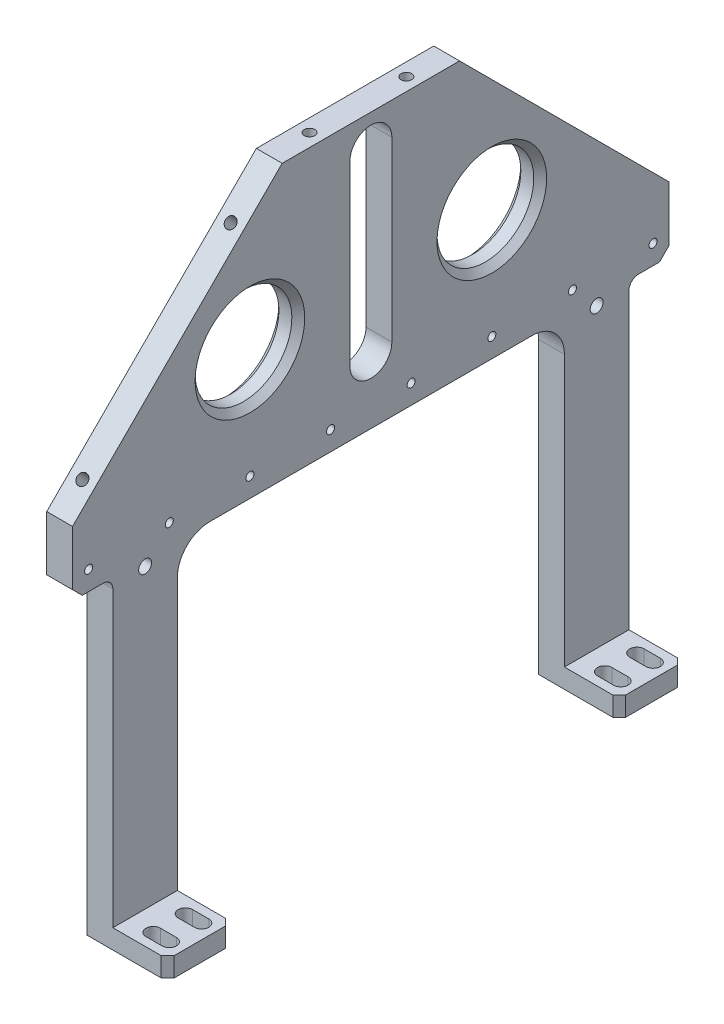
from build123d import *

# Parameters (mm, degrees)
BOSS_EXTRUDE1_DEPTH        = 92.5
CUT_EXTRUDE5_DEPTH         = 209.3416665
M4_TAPPED_HOLE1_D          = 3.3
M4_TAPPED_HOLE1_DEPTH      = 10.1
M4_TAPPED_HOLE1_TIP        = 0.991420021
SKETCH19_W                 = 12.5
SKETCH19_H                 = 100
CUT_EXTRUDE6_DEPTH         = 209.3416665
SKETCH10_R                 = 15
SKETCH10_W                 = 120
SKETCH10_H                 = 100
CUT_EXTRUDE3_DEPTH         = 209.3416665
M3_TAPPED_HOLE1_D          = 2.5
SIZE_MM_BLIND_PIN_HOLE1_D  = 4
CUT_EXTRUDE7_DEPTH         = 209.3416665
CHAMFER2_SIZE              = 65
CHAMFER3_SIZE              = 3
CHAMFER4_SIZE              = 2
FILLET1_R                  = 10
FILLET2_R                  = 3
M4_TAPPED_HOLE2_AT_2_COUNT = 2
M4_TAPPED_HOLE2_AT_2_PITCH = 65


with BuildPart() as part:
    # Sketch1 → Boss-Extrude1 (new, symmetric)
    with BuildSketch(Plane.XY):
        Polygon((0, 0), (25, 0), (25, 6), (8, 6), (8, 185), (0, 185), align=None)
    extrude(amount=BOSS_EXTRUDE1_DEPTH, both=True)

    # Sketch16 → Cut-Extrude5 (cut, through all)
    with BuildSketch(Plane.ZY):
        with BuildLine():
            Line((6.5, 175), (6.5, 120))
            ThreePointArc((6.5, 120), (0, 113.5), (-6.5, 120))
            Line((-6.5, 120), (-6.5, 175))
            ThreePointArc((-6.5, 175), (0, 181.5), (6.5, 175))
        make_face()
    extrude(amount=-CUT_EXTRUDE5_DEPTH, mode=Mode.SUBTRACT)

    # M4 Tapped Hole1
    with Locations(Plane(origin=(0, 185, 0), x_dir=(1, 0, 0), z_dir=(0, 1, 0))):
        with Locations((4, 15), (4, -15)):
            Hole(M4_TAPPED_HOLE1_D / 2, depth=M4_TAPPED_HOLE1_DEPTH)
            with Locations((0, 0, -(M4_TAPPED_HOLE1_DEPTH + M4_TAPPED_HOLE1_TIP / 2))):  # 118° drill point
                Cone(0, M4_TAPPED_HOLE1_D / 2, M4_TAPPED_HOLE1_TIP, mode=Mode.SUBTRACT)

    # Sketch19 → Cut-Extrude6 (cut, through all)
    with BuildSketch(Plane.ZY):
        with Locations((86.25, 50)):
            Rectangle(SKETCH19_W, SKETCH19_H)
        with Locations((-86.25, 50)):
            Rectangle(SKETCH19_W, SKETCH19_H)
    extrude(amount=-CUT_EXTRUDE6_DEPTH, mode=Mode.SUBTRACT)

    # Sketch10 → Cut-Extrude3 (cut, through all)
    with BuildSketch(Plane.ZY):
        with Locations((37.5, 140)):
            Circle(SKETCH10_R)
        with Locations((-37.5, 140)):
            Circle(SKETCH10_R)
        with Locations((0, 50)):
            Rectangle(SKETCH10_W, SKETCH10_H)
    extrude(amount=-CUT_EXTRUDE3_DEPTH, mode=Mode.SUBTRACT)

    # M3 Tapped Hole1 (through all)
    with Locations(Plane.ZY):
        with Locations((-87.5, 106), (-62.5, 106), (-37.5, 106), (-12.5, 106), (12.5, 106), (37.5, 106), (62.5, 106), (87.5, 106)):
            Hole(M3_TAPPED_HOLE1_D / 2)

    # Size mm Blind Pin Hole1 (through all)
    with Locations(Plane.ZY):
        with Locations((-70, 98), (70, 98)):
            Hole(SIZE_MM_BLIND_PIN_HOLE1_D / 2)

    # Sketch25 → Cut-Extrude7 (cut, through all)
    with BuildSketch(Plane.XZ):
        with BuildLine():
            Line((20.5, 72.75), (15.5, 72.75))
            ThreePointArc((15.5, 72.75), (13.25, 75), (15.5, 77.25))
            Line((15.5, 77.25), (20.5, 77.25))
            ThreePointArc((20.5, 77.25), (22.75, 75), (20.5, 72.75))
        make_face()
        with BuildLine():
            Line((20.5, 62.75), (15.5, 62.75))
            ThreePointArc((15.5, 62.75), (13.25, 65), (15.5, 67.25))
            Line((15.5, 67.25), (20.5, 67.25))
            ThreePointArc((20.5, 67.25), (22.75, 65), (20.5, 62.75))
        make_face()
        with BuildLine():
            Line((20.5, -67.25), (15.5, -67.25))
            ThreePointArc((15.5, -67.25), (13.25, -65), (15.5, -62.75))
            Line((15.5, -62.75), (20.5, -62.75))
            ThreePointArc((20.5, -62.75), (22.75, -65), (20.5, -67.25))
        make_face()
        with BuildLine():
            Line((20.5, -77.25), (15.5, -77.25))
            ThreePointArc((15.5, -77.25), (13.25, -75), (15.5, -72.75))
            Line((15.5, -72.75), (20.5, -72.75))
            ThreePointArc((20.5, -72.75), (22.75, -75), (20.5, -77.25))
        make_face()
    extrude(amount=-CUT_EXTRUDE7_DEPTH, mode=Mode.SUBTRACT)

    # Chamfer2
    chamfer2_edges = [part.edges().sort_by_distance(p)[0] for p in [
        (4, 185, 92.5),
        (4, 185, -92.5),
    ]]
    chamfer(chamfer2_edges, length=CHAMFER2_SIZE)

    # Chamfer3
    chamfer3_edges = [part.edges().sort_by_distance(p)[0] for p in [
        (4, 100, 92.5),
        (4, 100, -92.5),
    ]]
    chamfer(chamfer3_edges, length=CHAMFER3_SIZE)

    # Chamfer4
    chamfer4_edges = [part.edges().sort_by_distance(p)[0] for p in [
        (8, 140, 22.5),
        (0, 140, 22.5),
        (8, 140, -52.5),
        (0, 140, -52.5),
        (25, 3, 80),
        (25, 3, -80),
        (25, 3, -60),
        (25, 3, 60),
    ]]
    chamfer(chamfer4_edges, length=CHAMFER4_SIZE)

    # Fillet1
    fillet1_edges = [part.edges().sort_by_distance(p)[0] for p in [
        (4, 100, -60),
        (4, 100, 60),
    ]]
    fillet(fillet1_edges, radius=FILLET1_R)

    # Fillet2
    fillet2_edges = [part.edges().sort_by_distance(p)[0] for p in [
        (4, 100, 80),
        (4, 100, -80),
    ]]
    fillet(fillet2_edges, radius=FILLET2_R)

    # Sketch26 → M4 Tapped Hole2 (revolve, cut)
    with BuildSketch(Plane(origin=(4, 173.033008589, -39.466991411), x_dir=(0, 0.7071067811865487, 0.7071067811865465), z_dir=(1, 0, 0))):
        Polygon((0, 0), (0, 11.091420021), (1.65, 10.1), (1.65, 0), align=None)
    m4_tapped_hole2 = revolve(axis=Axis((4, 177.52313665, -43.957119472), (0, -0.7071067811865465, 0.7071067811865486)), mode=Mode.SUBTRACT)

    # M4 Tapped Hole2 at 2: M4 Tapped Hole2 ×2
    with Locations(*[Vector(0, -0.7071067811865485, -0.7071067811865466) * (i * M4_TAPPED_HOLE2_AT_2_PITCH) for i in range(1, M4_TAPPED_HOLE2_AT_2_COUNT)]):
        add(m4_tapped_hole2, mode=Mode.SUBTRACT)

    # Mirror1: M4 Tapped Hole2 across plane
    add(m4_tapped_hole2.mirror(Plane.XY), mode=Mode.SUBTRACT)

    # Mirror1 copy 1 sketch → Mirror1 copy 1 (revolve, cut)
    with BuildSketch(Plane(origin=(4, 127.071067812, 85.428932188), x_dir=(0, 0.7071067811865487, -0.7071067811865465), z_dir=(1, 0, 0))):
        Polygon((0, 0), (0, -11.091420021), (1.65, -10.1), (1.65, 0), align=None)
    revolve(axis=Axis((4, 131.561195872, 89.919060249), (0, 0.7071067811865465, 0.7071067811865486)), mode=Mode.SUBTRACT)


solid = part.part
